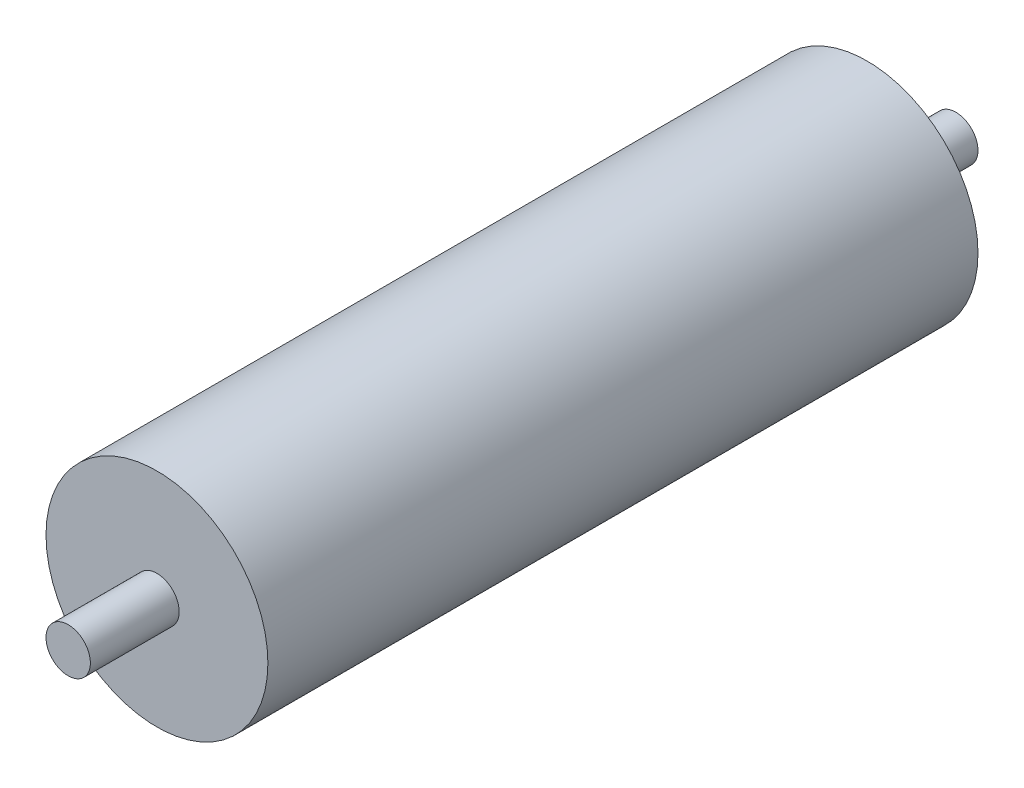
from build123d import *

# Parameters (mm, degrees)
SKETCH1_R           = 25
BOSS_EXTRUDE1_DEPTH = 160
SKETCH2_R           = 5
BOSS_EXTRUDE2_DEPTH = 20


with BuildPart() as part:
    # Sketch1 → Boss-Extrude1 (new body)
    with BuildSketch(Plane.XY):
        Circle(SKETCH1_R)
    extrude(amount=BOSS_EXTRUDE1_DEPTH)

    # Sketch2 → Boss-Extrude2 (add)
    with BuildSketch(Plane(origin=(0, 0, 0), x_dir=(-1, 0, 0), z_dir=(0, 0, -1))):
        Circle(SKETCH2_R)
    boss_extrude2 = extrude(amount=BOSS_EXTRUDE2_DEPTH)

    # Mirror1: Boss-Extrude2 across plane
    add(boss_extrude2.mirror(Plane(origin=(0, 0, 80), x_dir=(1, 0, 0), z_dir=(0, 0, -1))))


solid = part.part
